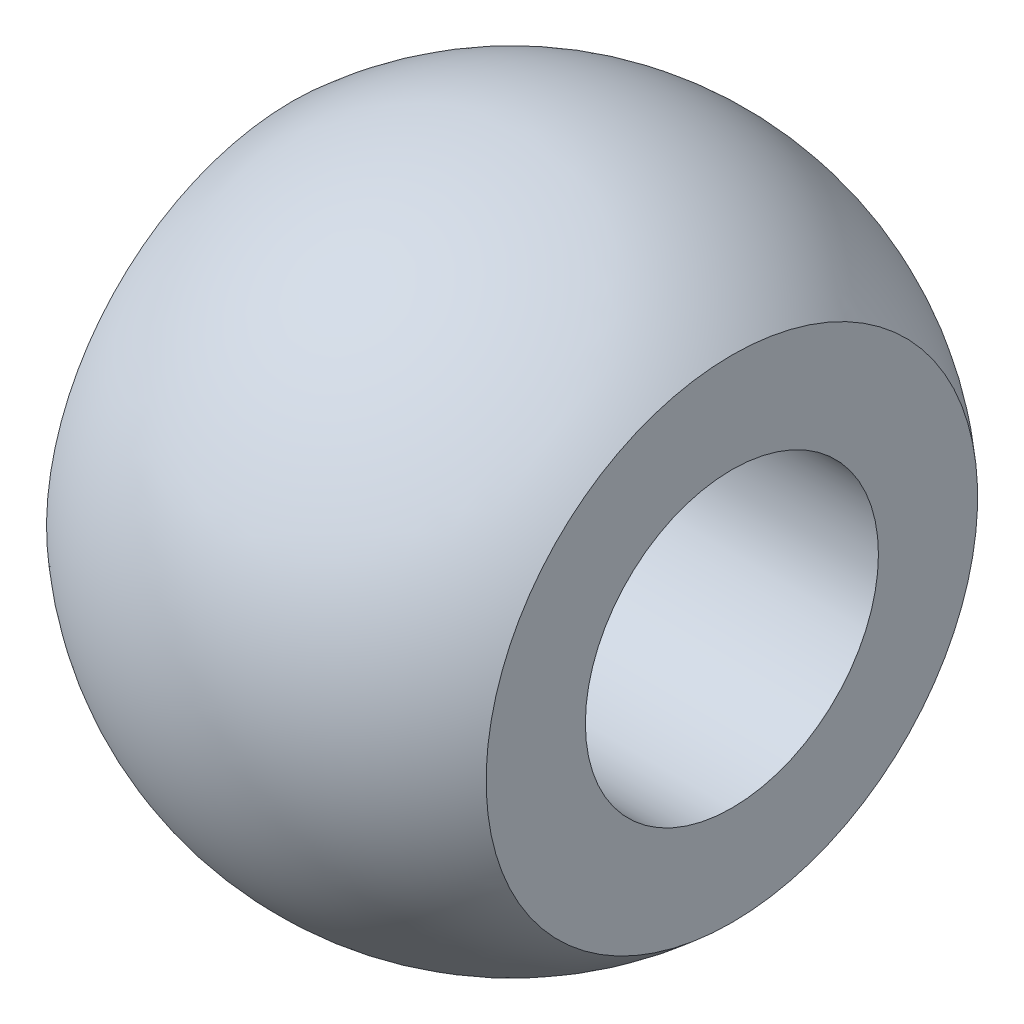
SolidWorks part; units mm, degrees
ref_plane "Front Plane" through (0, 0, 0) normal (0, 0, 1) x (1, 0, 0)
ref_plane "Top Plane" through (0, 0, 0) normal (0, 1, 0) x (1, 0, 0)
ref_plane "Right Plane" through (0, 0, 0) normal (1, 0, 0) x (0, 0, -1)
sketch "Sketch1" plane through (0, 0, 0) normal (0, 0, 1) x (1, 0, 0)
  line L0 (0, 4.5) -> (0, -4.5)
  arc A0 (0, -4.5) -> (0, 4.5) centre (0, 0) ccw
  dimension "D1" = 9
revolve "Revolve4" add sketch "Sketch1" angle 360 about L0
sketch "Sketch4" plane through (0, 0, 0) normal (0, 0, 1) x (1, 0, 0)
  line L0 (0, 4.2558) -> (0, -4.2141) construction
  line L1 (7.7375, 4.6179) -> (3, 4.6179)
  line L2 (7.7375, 4.6179) -> (7.7375, -4.6541)
  line L3 (7.7375, -4.6541) -> (3, -4.6541)
  line L4 (3, 4.6179) -> (3, -4.6541)
  line L5 (-3, 4.6179) -> (-3, -4.6541)
  line L6 (-7.7375, -4.6541) -> (-3, -4.6541)
  line L7 (-7.7375, 4.6179) -> (-7.7375, -4.6541)
  line L8 (-7.7375, 4.6179) -> (-3, 4.6179)
  dimension "D1" = 3
extrude "Cut-Extrude2" cut sketch "Sketch4" against normal mid plane 20
sketch "Sketch5" plane through (-3, 0, 0) normal (-1, 0, 0) x (0, 0, 1)
  circle A0 centre (0, 0) radius 2
  dimension "D1" = 4
extrude "Cut-Extrude3" cut sketch "Sketch5" against normal blind 20
